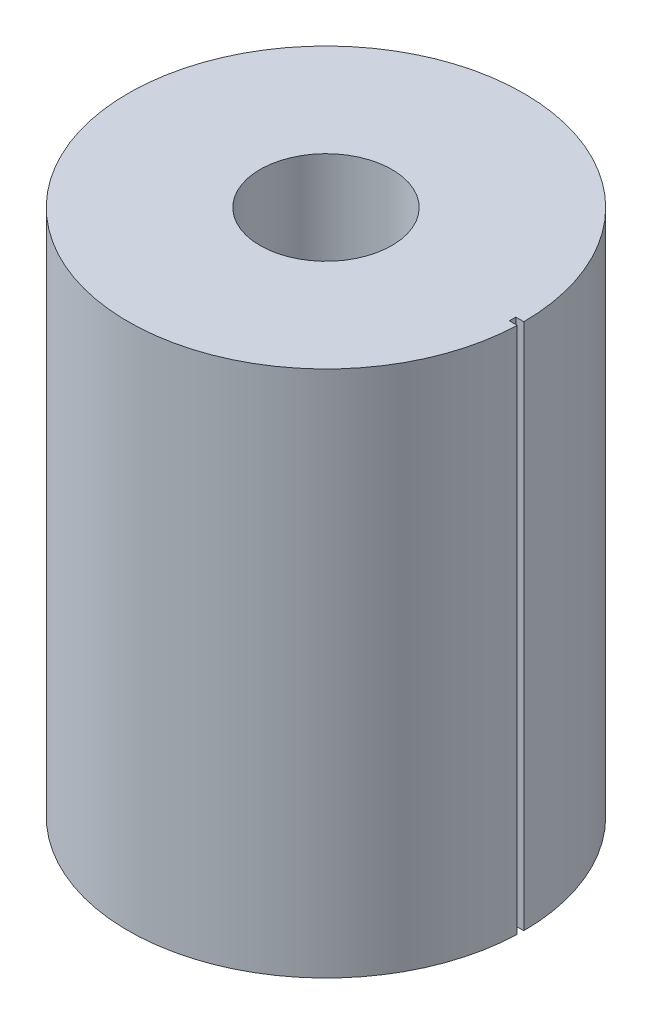
SolidWorks part; units mm, degrees
ref_plane "Front Plane" through (0, 0, 0) normal (0, 0, 1) x (1, 0, 0)
ref_plane "Top Plane" through (0, 0, 0) normal (0, 1, 0) x (1, 0, 0)
ref_plane "Right Plane" through (0, 0, 0) normal (1, 0, 0) x (0, 0, -1)
sketch "Sketch1" plane through (0, 0, 0) normal (0, 1, 0) x (1, 0, 0)
  circle A0 centre (0, 0) radius 7.5
  circle A1 centre (0, 0) radius 2.5
  dimension "D1" = 15
  dimension "D2" = 5
extrude "Boss-Extrude1" add sketch "Sketch1" along normal blind 20
sketch "Sketch2" plane through (0, 20, 0) normal (0, 1, 0) x (1, 0, 0)
  line L1 (7.1977, -0.2452) -> (7.8003, -0.2452)
  line L2 (7.1977, -0.2452) -> (7.1977, 0)
  line L3 (7.1977, 0) -> (7.8003, 0)
  line L4 (7.8003, -0.2452) -> (7.8003, 0)
  line L5 (7.1977, -0.2452) -> (7.8003, 0) construction
  line L6 (7.1977, 0) -> (7.8003, -0.2452) construction
  circle A0 centre (0, 0) radius 7.5 construction
  point P0 (7.499, -0.1226)
extrude "Cut-Extrude1" cut sketch "Sketch2" against normal through all
